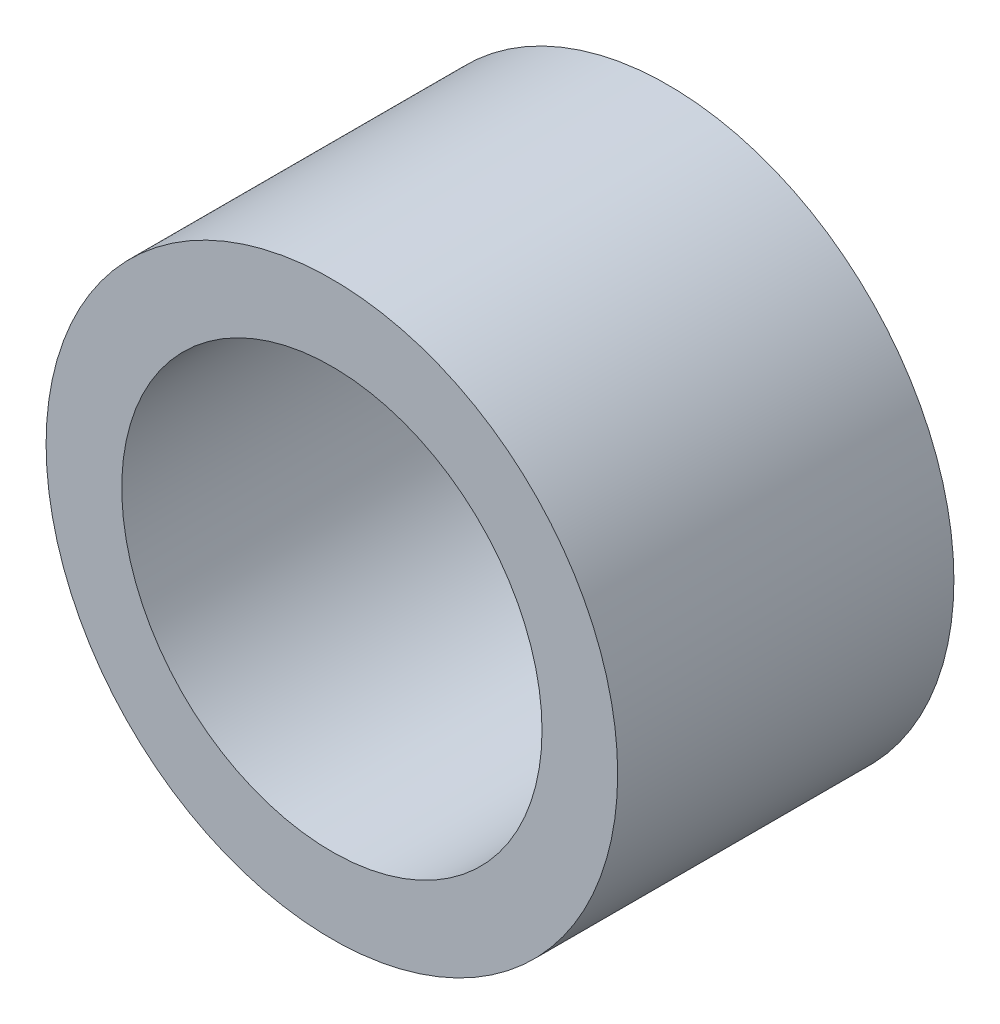
SolidWorks part; units mm, degrees
ref_plane "前视基准面" through (0, 0, 0) normal (0, 0, 1) x (1, 0, 0)
ref_plane "上视基准面" through (0, 0, 0) normal (0, 1, 0) x (1, 0, 0)
ref_plane "右视基准面" through (0, 0, 0) normal (1, 0, 0) x (0, 0, -1)
sketch "草图1" plane through (0, 0, 0) normal (0, 0, 1) x (1, 0, 0)
  circle A0 centre (0, 0) radius 6.25
  circle A1 centre (0, 0) radius 8.5
  dimension "D1" = 12.5
  dimension "D2" = 17
extrude "凸台-拉伸1" add sketch "草图1" along normal blind 10
